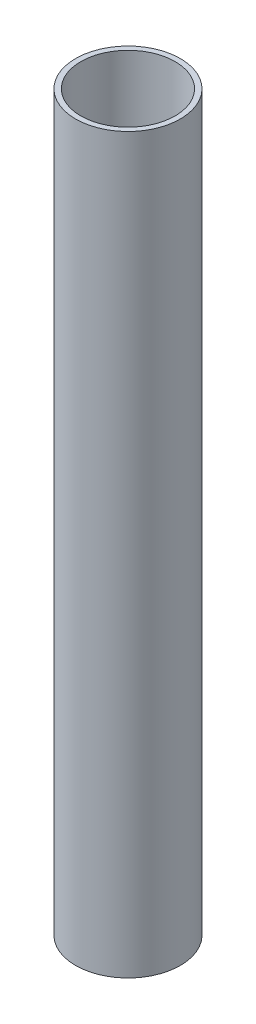
from build123d import *

# Parameters (mm, degrees)
SKETCH_1_R      = 10
SKETCH_1_R_2    = 9
EXTRUDE_1_DEPTH = 140


with BuildPart() as part:
    # 草图1 → 凸台-拉伸1 (new body)
    with BuildSketch(Plane(origin=(0, 0, 0), x_dir=(1, 0, 0), z_dir=(0, 1, 0))):
        with Locations(Location((0, 0, 0), (0, 0, 270))):
            Circle(SKETCH_1_R)
        with Locations(Location((0, 0, 0), (0, 0, 270))):
            Circle(SKETCH_1_R_2, mode=Mode.SUBTRACT)
    extrude(amount=EXTRUDE_1_DEPTH)


solid = part.part
